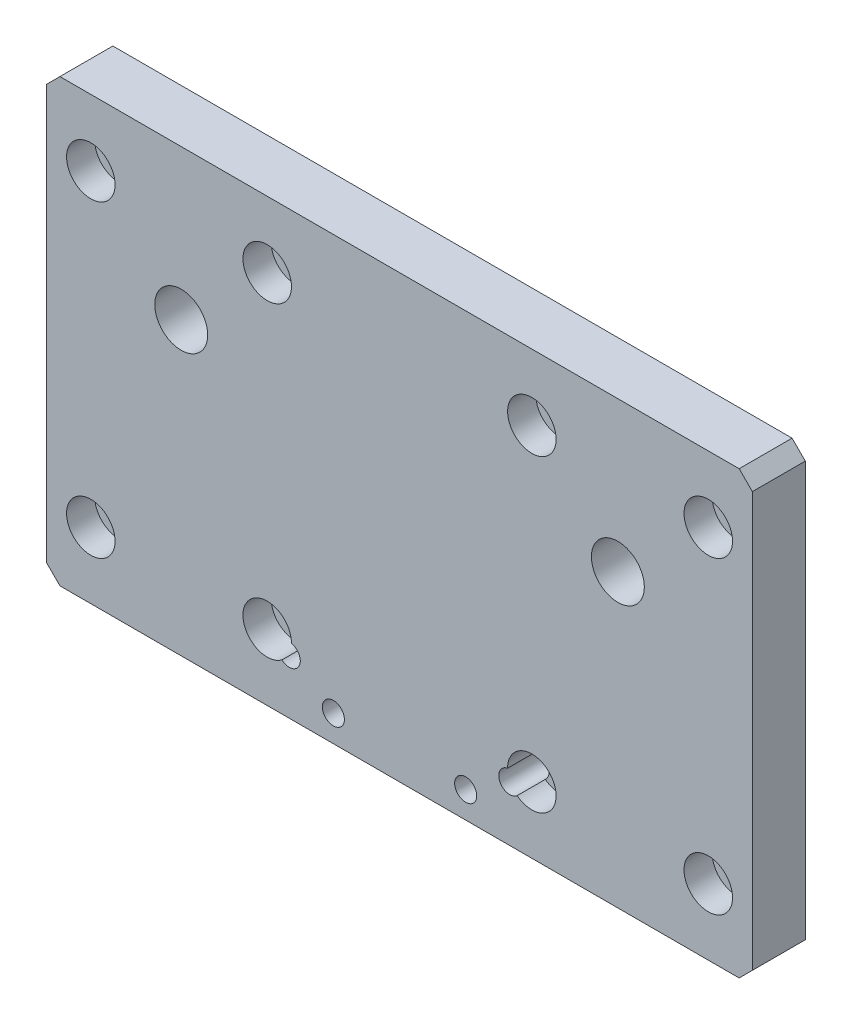
from build123d import *

# Parameters (mm, degrees)
SKETCH_1_W                   = 160
SKETCH_1_H                   = 100
EXTRUDE_1_DEPTH              = 12
HOLE_WIZARD_M14_1_D          = 12
HOLE_WIZARD_M6_1_D           = 6.4
HOLE_WIZARD_M6_1_CBORE_D     = 11
HOLE_WIZARD_M6_1_CBORE_DEPTH = 6.4
CHAMFER_1_SIZE               = 3
HOLE_WIZARD_M6_1_2_D         = 5
HOLE_WIZARD_M6_2_D           = 5
HOLE_WIZARD_M6_2_DEPTH       = 15
HOLE_WIZARD_M6_2_TIP         = 1.502151548


with BuildPart() as part:
    # 草图1 → 凸台-拉伸1 (new body)
    with BuildSketch(Plane.XY):
        with Locations((80, 50)):
            Rectangle(SKETCH_1_W, SKETCH_1_H)
    extrude(amount=EXTRUDE_1_DEPTH)

    # M14 螺纹孔1 (through all)
    with Locations(Plane.XY.offset(12)):
        with Locations((30.5, 66), (129.5, 66)):
            Hole(HOLE_WIZARD_M14_1_D / 2)

    # Hole Wizard M6 _1 (through all)
    with Locations(Plane.XY.offset(12)):
        with Locations((10, 15), (50, 15), (50, 85), (10, 85), (110, 15), (150, 15), (150, 85), (110, 85)):
            CounterBoreHole(HOLE_WIZARD_M6_1_D / 2, HOLE_WIZARD_M6_1_CBORE_D / 2, HOLE_WIZARD_M6_1_CBORE_DEPTH)

    # 倒角1
    chamfer_1_edges = [part.edges().sort_by_distance(p)[0] for p in [
        (0, 100, 6),
        (160, 100, 6),
        (160, 0, 6),
        (0, 0, 6),
    ]]
    chamfer(chamfer_1_edges, length=CHAMFER_1_SIZE)

    # Hole Wizard M6 _1 2 (through all)
    with Locations(Plane(origin=(0, 0, 0), x_dir=(-1, 0, 0), z_dir=(0, 0, -1))):
        with Locations((-65, 6), (-95, 6)):
            Hole(HOLE_WIZARD_M6_1_2_D / 2)

    # M6 螺纹孔2
    with Locations(Plane.XY.offset(12)):
        with Locations((55, 12.5), (105, 12.5)):
            Hole(HOLE_WIZARD_M6_2_D / 2, depth=HOLE_WIZARD_M6_2_DEPTH)
            with Locations((0, 0, -(HOLE_WIZARD_M6_2_DEPTH + HOLE_WIZARD_M6_2_TIP / 2))):  # 118° drill point
                Cone(0, HOLE_WIZARD_M6_2_D / 2, HOLE_WIZARD_M6_2_TIP, mode=Mode.SUBTRACT)


solid = part.part
